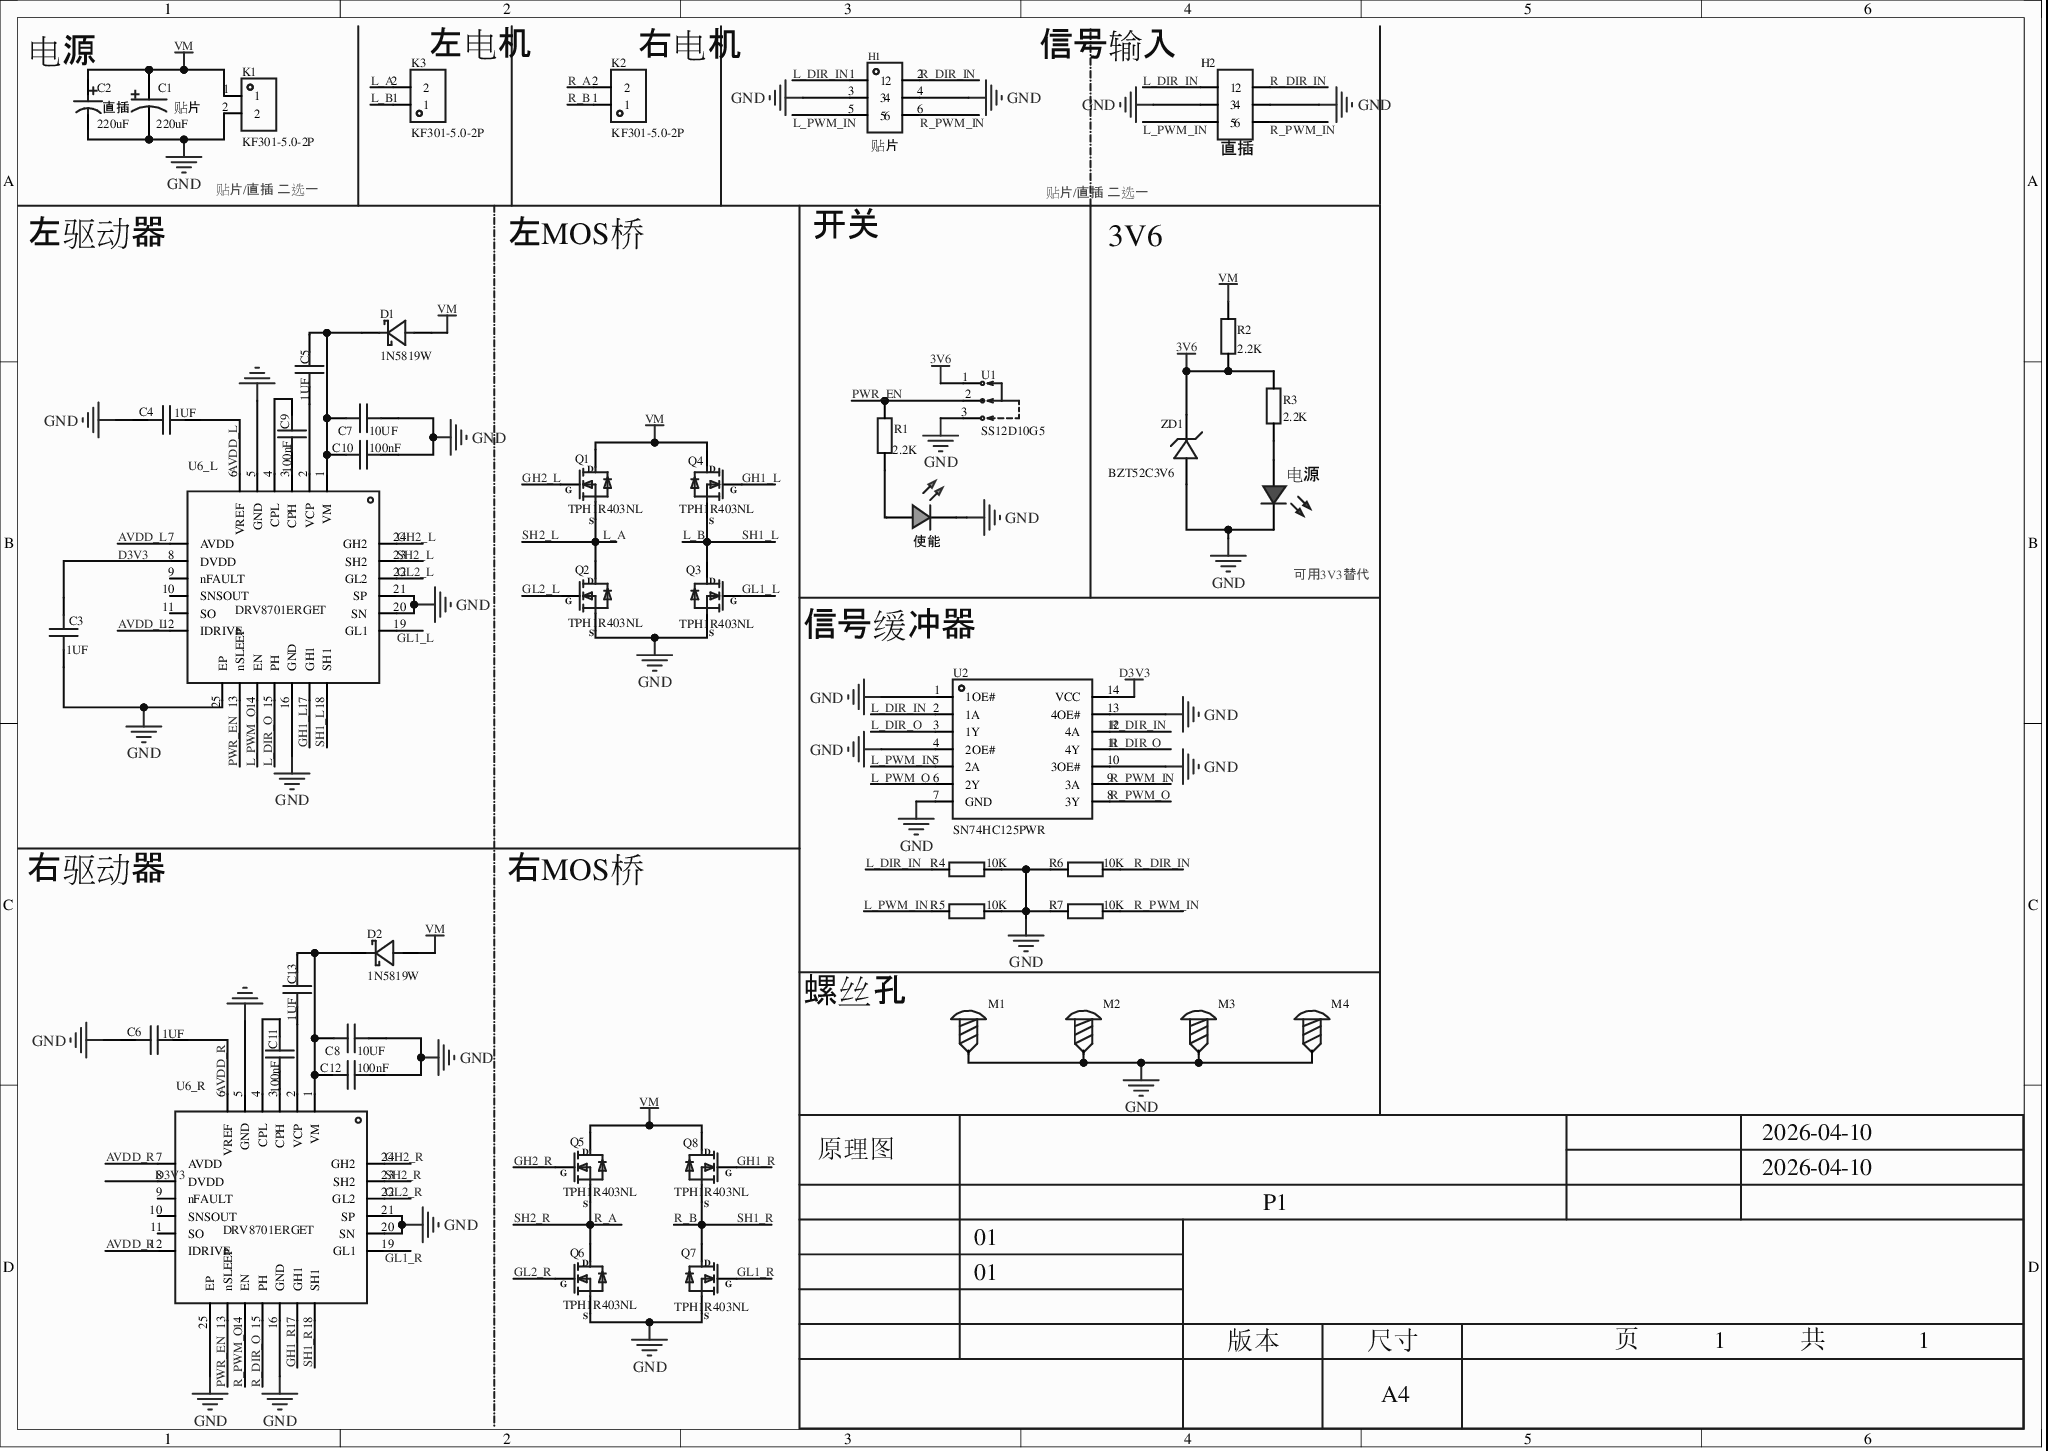
[diagram p0: MISC49921-3.schdoc]
# Altium project MISC49921-2.PrjPcb
1 sheet, 46 parts. Net scope: global (net labels, ports and power ports of the same name join across sheets).
Board file: MISC49921.pcbdoc

## Sheet MISC49921-3.schdoc
size 297 x 210 mm; Version: V1.0; @Project Name: MISC49921; @Page Count: 1; @Update Date: 2026-04-10; @Create Date: 2026-04-10; @Schematic Name: MISC49921; @Page No: 1; @Board Name: MISC49921; @Create Time: 08:46:51; @Update Time: 16:46:51

### Parts
C1  220uF  [CAP-SMD_BD8.0-L8.3-W8.3-FD]
C2  220uF  [CAP-TH_BD8.0-P3.50-D0.6-FD]
C3  1UF  [C0603]
C4  1UF  [C0603]
C5  1UF  [C0603]
C6  1UF  [C0603]
C7  10UF  [C0603]
C8  10UF  [C0603]
C9  100nF  [C0603]
C10  100nF  [C0603]
C11  100nF  [C0603]
C12  100nF  [C0603]
C13  1UF  [C0603]
D1  1N5819W  [SOD-123_L2.7-W1.6-LS3.7-RD-1]
D2  1N5819W  [SOD-123_L2.7-W1.6-LS3.7-RD-1]
H1  贴片  [HDR-SMD_6P-P2.54-V-M-R2-C5-S7.4]
H2  (no value)  [HDR-TH_6P-P2.54-V-R2-C3-S2.54_A2541WV-2X3P]
K1  KF301-5.0-2P  [CONN-TH_P5.00_KF301-5.0-2P]
K2  KF301-5.0-2P  [CONN-TH_P5.00_KF301-5.0-2P]
K3  KF301-5.0-2P  [CONN-TH_P5.00_KF301-5.0-2P]
M1  (no value)  [M4螺丝]
M2  (no value)  [M4螺丝]
M3  (no value)  [M4螺丝]
M4  (no value)  [M4螺丝]
Q1  TPH1R403NL  [DFN5x6]
Q2  TPH1R403NL  [DFN5x6]
Q3  TPH1R403NL  [DFN5x6]
Q4  TPH1R403NL  [DFN5x6]
Q5  TPH1R403NL  [DFN5x6]
Q6  TPH1R403NL  [DFN5x6]
Q7  TPH1R403NL  [DFN5x6]
Q8  TPH1R403NL  [DFN5x6]
R1  2.2K  [R0603]
R2  2.2K  [R0603]
R3  2.2K  [R0603]
R4  10K  [R0603]
R5  10K  [R0603]
R6  10K  [R0603]
R7  10K  [R0603]
U1  SS12D10G5  [SW-TH_SHOU-HAN_SS12D10G4]
U2  SN74HC125PWR  [TSSOP-14_L5.0-W4.4-P0.65-LS6.5-BL]
U6_L  DRV8701ERGET  [VQFN-24_L4.0-W4.0-P0.50-BL-EP2.5]
U6_R  DRV8701ERGET  [VQFN-24_L4.0-W4.0-P0.50-BL-EP2.5]
ZD1  BZT52C3V6  [SOD-123_L2.8-W1.8-LS3.7-RD]
使能  (no value)  [LED_0603]
电源  (no value)  [LED_0603]

### Nets
3V6: R2.1 R3.2 U1.1 ZD1.1(K)
D3V3: C3.2 U2.14(VCC) U6_L.8(DVDD) U6_R.8(DVDD)
GND: C1.2 C2.2 C3.1 C4.2 C6.2 C7.2 C8.2 C10.2 C12.2 H1.3 H1.4 H2.3 H2.4 K1.2 M1.1 M2.1 M3.1 M4.1 Q2.3(S) Q3.3(S) Q6.3(S) Q7.3(S) R4.2 R5.2 R6.1 R7.1 U1.3 U2.1(1OE#) U2.4(2OE#) U2.7(GND) U2.10(3OE#) U2.13(4OE#) U6_L.5(GND) U6_L.16(GND) U6_L.20(SN) U6_L.21(SP) U6_L.25(EP) U6_R.5(GND) U6_R.16(GND) U6_R.20(SN) U6_R.21(SP) U6_R.25(EP) ZD1.2(A) 使能.1(C) 电源.1(C)
VM: C1.1 C2.1 D1.2(A) D2.2(A) K1.1 Q1.1(D) Q4.1(D) Q5.1(D) Q8.1(D) R2.2
AVDD_L: C4.1 U6_L.6(VREF) U6_L.7(AVDD) U6_L.12(IDRIVE)
AVDD_R: C6.1 U6_R.6(VREF) U6_R.7(AVDD) U6_R.12(IDRIVE)
GH1_L: Q4.2(G) U6_L.17(GH1)
GH1_R: Q8.2(G) U6_R.17(GH1)
GH2_L: Q1.2(G) U6_L.24(GH2)
GH2_R: Q5.2(G) U6_R.24(GH2)
GL1_L: Q3.2(G) U6_L.19(GL1)
GL1_R: Q7.2(G) U6_R.19(GL1)
GL2_L: Q2.2(G) U6_L.22(GL2)
GL2_R: Q6.2(G) U6_R.22(GL2)
L_A: K3.2 Q1.3(S) Q2.1(D) U6_L.23(SH2)  [also labelled SH2_L]
L_B: K3.1 Q3.1(D) Q4.3(S) U6_L.18(SH1)  [also labelled SH1_L]
L_DIR_IN: H1.1 H2.1 R4.1 U2.2(1A)
L_DIR_O: U2.3(1Y) U6_L.15(PH)
L_PWM_IN: H1.5 H2.5 R5.1 U2.5(2A)
L_PWM_O: U2.6(2Y) U6_L.14(EN)
PWR_EN: R1.2 U1.2 U6_L.13(nSLEEP) U6_R.13(nSLEEP)
R_A: K2.2 Q5.3(S) Q6.1(D) U6_R.23(SH2)  [also labelled SH2_R]
R_B: K2.1 Q7.1(D) Q8.3(S) U6_R.18(SH1)  [also labelled SH1_R]
R_DIR_IN: H1.2 H2.2 R6.2 U2.12(4A)
R_DIR_O: U2.11(4Y) U6_R.15(PH)
R_PWM_IN: H1.6 H2.6 R7.2 U2.9(3A)
R_PWM_O: U2.8(3Y) U6_R.14(EN)
NetC5_1: C5.1 C7.1 C10.1 D1.1(K) U6_L.1(VM)
NetC5_2: C5.2 U6_L.2(VCP)
NetC8_1: C8.1 C12.1 C13.1 D2.1(K) U6_R.1(VM)
NetC9_1: C9.1 U6_L.3(CPH)
NetC9_2: C9.2 U6_L.4(CPL)
NetC11_1: C11.1 U6_R.3(CPH)
NetC11_2: C11.2 U6_R.4(CPL)
NetC13_2: C13.2 U6_R.2(VCP)
NetR1_1: R1.1 使能.2(A)
NetR3_1: R3.1 电源.2(A)

Not connected (* = marked no-connect by the designer): U6_L 9(nFAULT)* 10(SNSOUT)* 11(SO)*; U6_R 9(nFAULT)* 10(SNSOUT)* 11(SO)*

### Notes on the sheet
- (near C2) 电源
- (near K3) 左电机
- (near K2) 右电机
- 信号输入
- (near C2) 直插
- (near C1) 贴片
- (near H2) 直插
- 左驱动器
- 贴片/直插 二选一
- 左MOS桥
- 开关
- 3V6
- (near 电源) 可用3V3替代
- 信号缓冲器
- 右驱动器
- 右MOS桥
- 螺丝孔
- 2026-04-10
- 原理图
- P1
- 01
- 版本
- 尺寸
- A4
- 页
- 1
- 共

### Library data of the parts
C1 = EEEFT1H221GP: 容值:220uF;精度:±20%;额定电压:50V;纹波电流:670mA@100kHz;等效串联电阻:180mΩ@100kHz;; Manufacturer: PANASONIC(松下); AddInBom: yes; ModelId: 5c9301d64f8b45ea89e061ac72e6cbf7; ModelTransform: 393.7,326.771,0,180,0,0,0,0,0; Tolerance: ±20%; Rated Voltage: 50V; φD: 8mm; L: 10.5mm; Lifetime @ Temp: 5000hrs@105℃; Symbol: EEEFT1H221GP; Device: EEEFT1H221GP; Supplier: LCSC; Supplier Part: C178595; Manufacturer Part: EEEFT1H221GP; Value: 220uF; JLCPCB Part Class: 扩展库; LCSC Part Name: 220uF ±20% 50V; Supplier Footprint: SMD,D8xL10.2mm; Datasheet: https://atta.szlcsc.com/upload/public/pdf/source/20180420/C190724_5C30A39F6DC8D73DF4133310F276C40B.pdf; ConvertToPcb: yes; FootprintName: CAP-SMD_BD8.0-L8.3-W8.3-FD; ModelName: CAP-SMD_BD8.0-L8.3-W8.3-FD; Ripple Current: 670mA@100kHz; Equivalent Series Resistance(ESR): 180mΩ@100kHz; Operating Temperature: -55℃~+105℃
C2 = ERS1VM221F12OT: 容值:220uF;精度:±20%;额定电压:35V;; Manufacturer: AISHI(艾华集团); AddInBom: yes; ModelId: a2c936ec27754f809f3966430e36f767; ModelName: CAP-TH_D8.0-H8.0-P3.50; ModelTransform: 314.96,314.862,0,180,0,0,0,0,-137.795; Tolerance: ±20%; Rated Voltage: 35V; φD: 8mm; L: 12mm; Lifetime @ Temp: 7000hrs@105℃; Symbol: ERS1VM221F12OT; Device: ERS1VM221F12OT; LCSC Part Name: 220uF ±20% 35V; SupplierPart: C106697; ManufacturerPart: ERS1VM221F12OT; Supplier Footprint: 插件,D8xL12mm; JLCPCB Part Class: 扩展库; Datasheet: https://atta.szlcsc.com/upload/public/pdf/source/20191015/C438940_4B8E60A742BB0AE40DDEF87A5C89089D.pdf; Supplier: LCSC; ConvertToPcb: yes; FootprintName: CAP-TH_BD8.0-P3.50-D0.6-FD; Value: 220uF; Lead Spacing: 3.5mm
C3-C13 = CAP_0603: ConvertToPcb: yes; SymbolName: CapAcitance; ModelId: ac125912035d415993ca9572d50418b1; ModelName: C0603_L1.6-W0.8-H0.8; ModelTransform: 62.992,31.496,0,0,0,0,0,0,0; Device: CAP_0603; AddInBom: yes; Supplier Footprint: 0603; FootprintName: C0603
  C3-C6 C13: Value: 1UF
  C7 C8: Value: 10UF
  C9-C12: Value: 100nF
D1 D2 = 1N5819W: 二极管配置:-;正向压降(Vf):900mV@3A;直流反向耐压(Vr):40V;平均整流电流(Io):1A;; Manufacturer: TECH PUBLIC(台舟); Symbol: 1N5819W_C2905650; AddInBom: yes; ModelId: 528459655f7d4601a76356f3191c812b; ModelTransform: 151.575,66.929,0,0,0,0,0,0,0; Reverse Voltage (Vr): 40V; Average Rectified Current (Io): 1A; Reverse Leakage Current (Ir): 1mA@40V; Device: 1N5819W; LCSC Part Name: 电压:40V 电流:1A; SupplierPart: C2905650; ManufacturerPart: 1N5819W; Supplier Footprint: SOD-123; JLCPCB Part Class: 扩展库; Datasheet: https://atta.szlcsc.com/upload/public/pdf/source/20211020/7FEA34DA99E5285CBA3CC87767B82BE7.pdf; Supplier: LCSC; ConvertToPcb: yes; FootprintName: SOD-123_L2.7-W1.6-LS3.7-RD-1; ModelName: SOD-123_L2.7-W1.6-LS3.7-RD-1; Diode Configuration: -; Forward Voltage (Vf@If): 900mV@3A
H1 = 2.54-2*3P立贴针: 插针结构:-;间距:2.54mm;行距:-;圆针/方针:-;安装类型:-;排数:双排;总PIN位数:6P;额定电流:-;额定电压:-;配合针长度:-;塑高:-;触头材质:-;触头镀层:-;颜色:黑色;; Manufacturer: BOOMELE(博穆精密); AddInBom: yes; ModelId: 04f7a77b3a774fdf8b1caeaa3d5fc986; ModelName: HDR-SMD_6P-P2.54-M-LS-2X3P; ModelTransform: 299.9994,275.59,0,0,0,0,0,0.001,0; Pitch: 2.54mm; Manufacturer Part: 贴片; Symbol: 2.54-2*3P立贴针; Device: 2.54-2*3P立贴针; Supplier: LCSC; Supplier Part: C192301; JLCPCB Part Class: 扩展库; LCSC Part Name: 间距:2.54mm; Supplier Footprint: SMD,P=2.54mm,卧贴; ConvertToPcb: yes; FootprintName: HDR-SMD_6P-P2.54-V-M-R2-C5-S7.4; Pin Structure: -; Row Spacing: -; Circluar Pins/Square Pins: -; Mounting Type: -; Number of Rows: 双排; Number of Pins: 6P; Current Rating (Max): -; Voltage Rating (Max): -; Length of Mating Pin: -; Insulation Height: -; Contact Material: -; Contact Plating: -; Color: 黑色
H2 = HDR-M_2.54_2x3: Symbol: HDR-M-2.54_2x3; ConvertToPcb: yes; ModelId: fd1b55b786fb415ca65c4187088147b7; ModelName: HDR2.54-M-LI-2x3P; ModelTransform: 299.9994,200,0,0,0,0,0,0,-118.11; Device: HDR-M_2.54_2x3; AddInBom: yes; SupplierPart: C402781; Supplier Footprint: 插件,P=2.54mm; FootprintName: HDR-TH_6P-P2.54-V-R2-C3-S2.54_A2541WV-2X3P
K1 = KF301-5.0-2P: 结构:1x2P;间距:5mm;颜色:蓝色;安装方式:直插;额定电流:17A;额定电压:250V;排数:1;线规 - AWG:14~22;线规 - 平方毫米:1.5;每排PIN数:2;工作温度范围:-30℃~+120℃;; Manufacturer: KEFA(科发); AddInBom: yes; ModelId: 442de893d0fc4728b9e5c7abc29ccda5; ModelTransform: 409.448,303.149,0,0,0,0,7.874,5.906,-169.291; Structure: 1x2P; Pitch: 5mm; Current Rating (Max): 17A; Voltage Rating (Max): 250V; Wire Gauge - AWG: 14~22; Wire Gauge - mm2: 1.5; Number of PINs Per Row: 2; Symbol: KF301-5.0-2P; Device: KF301-5.0-2P; Supplier: LCSC; Supplier Part: C474881; Manufacturer Part: KF301-5.0-2P; JLCPCB Part Class: 扩展库; LCSC Part Name: 5mm 1x2P 排数:1 每排P数:2 直插; Supplier Footprint: 插件,P=5mm; Datasheet: https://atta.szlcsc.com/upload/public/pdf/source/20230317/03A5B5FC229D6F9225E8F51DA1A4E80A.pdf; ConvertToPcb: yes; FootprintName: CONN-TH_P5.00_KF301-5.0-2P; ModelName: CONN-TH_P5.00_KF301-5.0-2P; Color: 蓝色; Mounting Style: 直插; Number of Pins: 2P; Number of Rows: 1; Operating Temperature Range: -30℃~+120℃
K2 K3 = KF301-5.0-2P: 结构:1x2P;间距:5mm;颜色:蓝色;安装方式:直插;额定电流:17A;额定电压:250V;排数:1;线规 - AWG:14~22;线规 - 平方毫米:1.5;每排PIN数:2;工作温度范围:-30℃~+120℃;; Manufacturer: KEFA(科发); 3D Model: 442de893d0fc4728b9e5c7abc29ccda5; 3D Model Transform: 409.448,303.149,0,0,0,0,7.874,5.906,-169.291; Structure: 1x2P; Pitch: 5mm; Current Rating (Max): 17A; Voltage Rating (Max): 250V; Wire Gauge - AWG: 14~22; Wire Gauge - mm2: 1.5; Number of PINs Per Row: 2; AddInBom: yes; Symbol: KF301-5.0-2P; Device: KF301-5.0-2P; LCSC Part Name: 5mm 1x2P 排数:1 每排P数:2 直插; Supplier Footprint: 插件,P=5mm; Datasheet: https://atta.szlcsc.com/upload/public/pdf/source/20230317/03A5B5FC229D6F9225E8F51DA1A4E80A.pdf; Color: 蓝色; Mounting Style: 直插; Number of Pins: 2P; Number of Rows: 1; Operating Temperature Range: -30℃~+120℃; Supplier: LCSC; Supplier Part: C474881; Manufacturer Part: KF301-5.0-2P; JLCPCB Part Class: 扩展库; ConvertToPcb: yes; FootprintName: CONN-TH_P5.00_KF301-5.0-2P; ModelName: CONN-TH_P5.00_KF301-5.0-2P
M1-M4 = M4螺丝: Symbol: 螺丝孔; ConvertToPcb: yes; Device: M4螺丝; AddInBom: yes; Supplier Footprint: 插件; FootprintName: M4螺丝
Q1-Q8 = TPH1R403NL: AddInBom: yes; ModelId: 2220501111284f4fa264999823e2c1e0; ModelName: PDFN5x6; ModelTransform: 196.85,238.1884981226921,38.97630096212029,0,0,0,0,0,0; Device: TPH1R403NL; ConvertToPcb: yes; SymbolName: TPH1R403NL
R1-R7 = Res_0603: Symbol: 电阻; ConvertToPcb: yes; ModelId: fc143cca1e79419f9cd78b61e9279f08; ModelTransform: 31.8897,63.7794,0,90,0,0,0,0,0; Device: Res_0603; AddInBom: yes; Supplier Footprint: 0603; FootprintName: R0603; ModelName: R0603
  R1-R3: Value: 2.2K
  R4-R7: Value: 10K
U1 = SS12D10G5: 电路结构:单刀双掷;安装方式:直插;额定电流(DC):2A;额定电压(DC):125V;机械寿命:3千次;; Manufacturer: SHOU HAN(首韩); AddInBom: yes; ModelId: cfce8581009a45839cc96a3fa85751f8; ModelTransform: 499.999,263.779,0,0,0,0,-0.589,-0.591,-196.85; Circuit: 单刀双掷; Switch Length: 12.7mm; Switch Width: 6.7mm; Current Rating (DC): 2A; Voltage Rating (DC): 125V; Mechanical Life: 3千次; Symbol: SS12D10G5; Device: SS12D10G5; LCSC Part Name: 两档立式插件 3脚拨动开关 柄长5.0mm; SupplierPart: C7431054; ManufacturerPart: SS12D10G5; Supplier Footprint: 插件; JLCPCB Part Class: 扩展库; Datasheet: https://atta.szlcsc.com/upload/public/pdf/source/20231130/7A3DB6A149BF0A1DCFFE64FFC07FE434.pdf; Supplier: LCSC; ConvertToPcb: yes; FootprintName: SW-TH_SHOU-HAN_SS12D10G4; ModelName: SW-TH_SHOU-HAN_SS12D10G4; Mounting Style: 直插; Operating Temperature: -25℃~+70℃
U2 = SN74HC125PWR: 输入类型:-;电源电压:2V~6V;元件数:4;每个元件位数:1;灌电流(IOL):7.8mA;拉电流(IOH):7.8mA;; Manufacturer: TI(德州仪器); AddInBom: yes; ModelId: 02f1f60386074b2ca8e111040ac061f2; ModelName: TSSOP-14_L5.0-W4.4-H1.0-LS6.4-P0.65; ModelTransform: 236.714,196.85,0,90,0,0,0,0,0; output type: 三态; Supply Voltage: 2V~6V; Number of Elements: 4; Number of Bits per Element: 1; Sink Current: 7.8mA; Logic Family: 74HC; Symbol: SN74HC125PWR; Device: SN74HC125PWR; LCSC Part Name: SN74HC125PWR; SupplierPart: C132994; ManufacturerPart: SN74HC125PWR; Supplier Footprint: TSSOP-14; JLCPCB Part Class: 扩展库; Datasheet: https://www.ti.com/cn/lit/gpn/sn74hc125; Supplier: LCSC; ConvertToPcb: yes; FootprintName: TSSOP-14_L5.0-W4.4-P0.65-LS6.5-BL; Input type: -; Source Current: 7.8mA; Operating Temperature: -40℃~+85℃
U6_L U6_R = DRV8701ERGET: DRV8701 47V H 桥智能栅极驱动器; Manufacturer: TI(德州仪器); AddInBom: yes; ModelId: 12827167658848359cc215f26847ede4; ModelName: VQFN-24_L4.0-W4.0-H1.0-P0.50-BL-EP2.5; ModelTransform: 157.48,157.48,0,90,0,0,-0.001,0.001,0; Symbol: DRV8701ERGET; Device: DRV8701ERGET; LCSC Part Name: 有刷直流电机驱动芯片 5.5V; SupplierPart: C132049; ManufacturerPart: DRV8701ERGET; Supplier Footprint: VQFN-24(4x4); JLCPCB Part Class: 扩展库; Datasheet: https://www.ti.com/cn/lit/gpn/drv8701; Supplier: LCSC; ConvertToPcb: yes; FootprintName: VQFN-24_L4.0-W4.0-P0.50-BL-EP2.5
ZD1 = BZT52C3V6_C2113: 二极管配置:独立式;稳压值(标称值):3.6V;稳压值(范围):3.4V~3.8V;功率:350mW;精度:-;; Manufacturer: CJ(江苏长电/长晶); AddInBom: yes; ModelId: 7884390a25fb4c08947731ebfba7e3f8; ModelTransform: 144.8816,62.992,0,0,0,0,0,0,0; Diode Configuration: 独立式; Zener Voltage (Nom): 3.6V; Reverse Leakage Current (Ir): 5uA@1V; Power Dissipation: 350mW; Zener Impedance (Zzt): 90Ω; Device: BZT52C3V6_C2113; Symbol: BZT52C3V6_C2113; LCSC Part Name: BZT52C3V6; SupplierPart: C2113; ManufacturerPart: BZT52C3V6; Supplier Footprint: SOD-123; JLCPCB Part Class: 扩展库; Datasheet: https://atta.szlcsc.com/upload/public/pdf/source/20140508/1457707057629.pdf; Supplier: LCSC; ConvertToPcb: yes; FootprintName: SOD-123_L2.8-W1.8-LS3.7-RD; ModelName: SOD-123_L2.8-W1.8-LS3.7-RD; Zener Voltage (Range): 3.4V~3.8V; Tolerance: -
使能 = LED_0603-G: Symbol: LED_G; Convert to PCB: yes; 3D Model: 8b5fcaf0229049f8a37a9c352bb0ca0a; 3D Model Transform: 63.1,31.6,23.7,0,0,0,0,0,0; ModelName: LED-0603_G; Device: LED_0603-G; Add into BOM: yes; Supplier Footprint: 0603; FootprintName: LED_0603
电源 = LED_0603-R: Symbol: LED_R; Convert to PCB: yes; 3D Model: dd8257b0d61a4cd7b68939a056e08095; 3D Model Transform: 58.72,29.4,22.03,0,0,0,0,0,0; ModelName: LED-0603_R; Device: LED_0603-R; Add into BOM: yes; Supplier Footprint: 0603; FootprintName: LED_0603